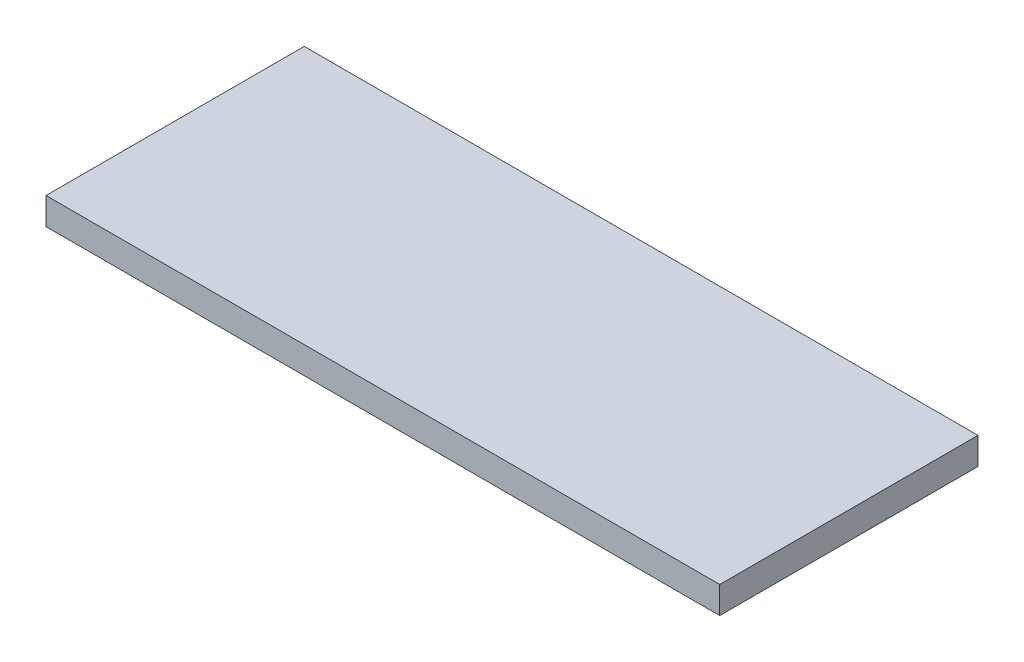
SolidWorks part; units mm, degrees
ref_plane "前视基准面" through (0, 0, 0) normal (0, 0, 1) x (1, 0, 0)
ref_plane "上视基准面" through (0, 0, 0) normal (0, 1, 0) x (1, 0, 0)
ref_plane "右视基准面" through (0, 0, 0) normal (1, 0, 0) x (0, 0, -1)
sketch "草图1" plane through (0, 0, 0) normal (0, 1, 0) x (1, 0, 0)
  line L1 (-150, -57.5) -> (150, -57.5)
  line L2 (-150, -57.5) -> (-150, 57.5)
  line L3 (-150, 57.5) -> (150, 57.5)
  line L4 (150, -57.5) -> (150, 57.5)
  line L5 (-150, -57.5) -> (150, 57.5) construction
  line L6 (-150, 57.5) -> (150, -57.5) construction
  point P0 (0, 0)
  dimension "D1" = 300
  dimension "D2" = 115
extrude "凸台-拉伸1" add sketch "草图1" along normal blind 12
